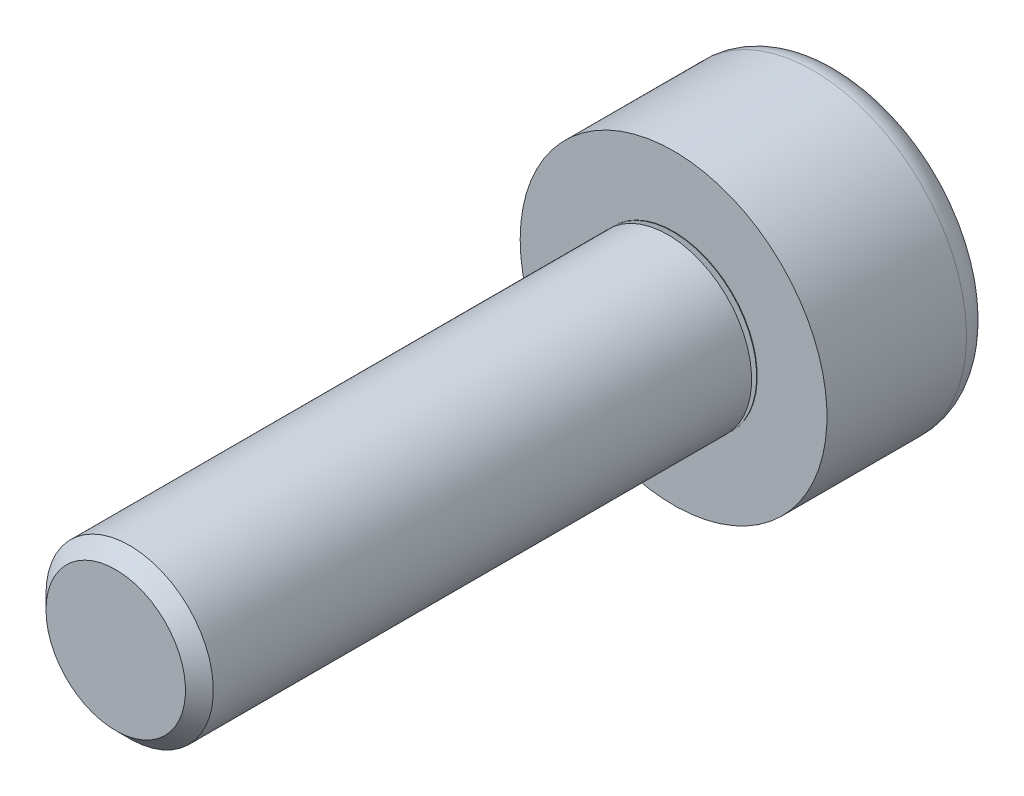
from build123d import *

# Parameters (mm, degrees)
CUT_EXTRUDE1_DEPTH = 1.25


with BuildPart() as part:
    # Logo3_bib1 → Revolve1 (revolve)
    with BuildSketch(Plane(origin=(0, 0, 0), x_dir=(-1, 0, 0), z_dir=(0, -1, 0))):
        with BuildLine():
            Line((0, -10), (0, 3))
            Line((0, 3), (2.25, 3))
            ThreePointArc((2.25, 3), (2.603553391, 2.853553391), (2.75, 2.5))
            Line((2.75, 2.5), (2.75, 0))
            Line((2.75, 0), (1.5, 0))
            Line((1.5, 0), (1.5, -0.01))
            Line((1.5, -0.01), (1.363425636, -0.01))
            ThreePointArc((1.363425636, -0.01), (1.343729481, -0.026527036), (1.356585234, -0.048793852))
            Line((1.356585234, -0.048793852), (1.5, -0.100992559))
            Line((1.5, -0.100992559), (1.5, -9.75))
            Line((1.5, -9.75), (1.25, -10))
            Line((1.25, -10), (0, -10))
        make_face()
    revolve(axis=Axis((0, 0, -10.585154653), (0, 0, 1)))

    # Logo3_bib2 → Cut-Extrude1 (cut)
    with BuildSketch(Plane(origin=(0, 0, -3), x_dir=(1, 0, 0), z_dir=(0, 0, -1))):
        Polygon((1.443375673, 0), (0.721687836, 1.25), (-0.721687836, 1.25), (-1.443375673, 0), (-0.721687836, -1.25), (0.721687836, -1.25), align=None)
    extrude(amount=-CUT_EXTRUDE1_DEPTH, mode=Mode.SUBTRACT)


solid = part.part
